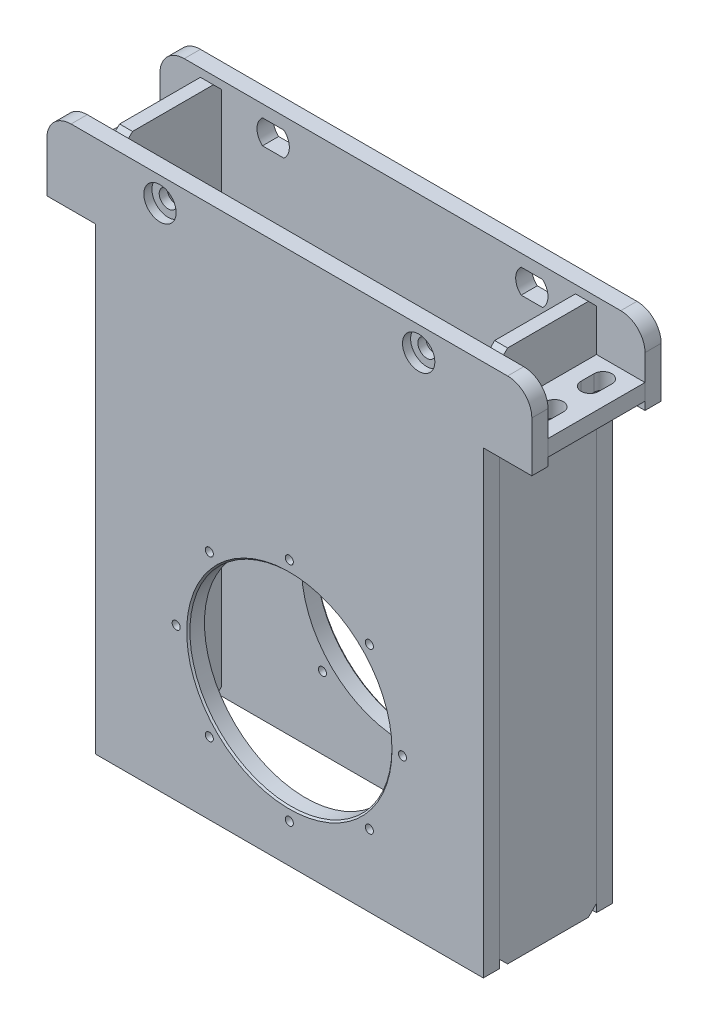
SolidWorks part; units mm, degrees
material "Plain carbon steel"
ref_plane "Front Plane" through (0, 0, 0) normal (0, 0, 1) x (1, 0, 0)
ref_plane "Top Plane" through (0, 0, 0) normal (0, 1, 0) x (1, 0, 0)
ref_plane "Right Plane" through (0, 0, 0) normal (1, 0, 0) x (0, 0, -1)
sketch "Sketch1" plane through (0, 0, 0) normal (0, 0, 1) x (1, 0, 0)
  line L1 (-150, 165) -> (150, 165)
  line L2 (-150, 165) -> (-150, -165)
  line L3 (-150, -165) -> (150, -165)
  line L4 (150, 165) -> (150, -165)
  line L5 (-150, 165) -> (150, -165) construction
  line L6 (-150, -165) -> (150, 165) construction
  point P0 (0, 0)
  dimension "D1" = 300
  dimension "D2" = 330
extrude "Boss-Extrude1" add sketch "Sketch1" along normal blind 10
sketch "Sketch2" plane through (0, 0, 10) normal (0, 0, 1) x (1, 0, 0)
  line L0 (150, 165) -> (-150, 165) construction
  circle A0 centre (-80, 150) radius 7.5
  dimension "D2" = 15
  dimension "D3" = 15
  dimension "D1" = 80
extrude "Cut-Extrude1" cut sketch "Sketch2" against normal blind 10
pattern_linear "LPattern1" count 2 spacing 160 along (1, 0, 0) of "Cut-Extrude1"
sketch "Sketch12" plane through (0, 0, 10) normal (0, 0, 1) x (1, 0, 0)
  line L0 (-150, -165) -> (150, -165) construction
  line L1 (120, -165) -> (112, -165)
  line L2 (120, -165) -> (120, 165)
  line L3 (120, 165) -> (112, 165)
  line L4 (112, -165) -> (112, 165)
  line L5 (-120, -165) -> (-112, -165)
  line L6 (-120, -165) -> (-120, 165)
  line L7 (-120, 165) -> (-112, 165)
  line L8 (-112, -165) -> (-112, 165)
  dimension "D1" = 330
  dimension "D2" = 8
  dimension "D3" = 8
  dimension "D4" = 330
  dimension "D5" = 120
  dimension "D6" = 120
extrude "Boss-Extrude2" add sketch "Sketch12" along normal blind 60 separate body
sketch "Sketch13" plane through (0, 0, 70) normal (0, 0, 1) x (1, 0, 0)
  line L0 (-150, 165) -> (-150, -165) construction
  line L1 (150, -165) -> (-150, -165)
  line L2 (150, -165) -> (150, 150)
  line L3 (135, 165) -> (-135, 165)
  line L4 (-150, -165) -> (-150, 150)
  arc A0 (150, 150) -> (135, 165) centre (135, 150) ccw
  arc A1 (-135, 165) -> (-150, 150) centre (-135, 150) ccw
  circle A2 centre (80, 150) radius 7.5 construction
  circle A3 centre (-80, 150) radius 7.5 construction
  circle A4 centre (80, 150) radius 7.5
  circle A5 centre (-80, 150) radius 7.5
  point P11 (-150, 165)
  dimension "D2" = 15
  dimension "D1" = 330
extrude "Boss-Extrude3" add sketch "Sketch13" along normal blind 10 separate body
sketch "Sketch14" plane through (120, 0, 0) normal (1, 0, 0) x (0, 0, -1)
  line L0 (-70, -165) -> (-70, 165) construction
  line L1 (-70, 124) -> (-10, 124)
  line L2 (-70, 124) -> (-70, 134)
  line L3 (-70, 134) -> (-10, 134)
  line L4 (-10, 124) -> (-10, 134)
  line L5 (-10, -165) -> (-10, 165) construction
  line L6 (-80, 165) -> (-70, 165) construction
  dimension "D1" = 10
  dimension "D2" = 31
extrude "Boss-Extrude4" add sketch "Sketch14" along normal blind 30 separate body
sketch "Sketch26" plane through (0, 134, 0) normal (0, 1, 0) x (1, 0, 0)
  line L0 (135, -10) -> (135, -70) construction
  line L1 (150, -10) -> (120, -10) construction
  line L2 (150, -70) -> (120, -70) construction
  line L3 (135, -40) -> (157.7954, -40) construction
  line L4 (135, -21) -> (135, -29) construction
  line L5 (140.5, -21) -> (140.5, -29)
  line L6 (129.5, -21) -> (129.5, -29)
  line L7 (135, -59) -> (135, -51) construction
  line L8 (129.5, -59) -> (129.5, -51)
  line L9 (140.5, -59) -> (140.5, -51)
  circle A0 centre (135, -25) radius 5.5 construction
  circle A1 centre (135, -55) radius 5.5 construction
  arc A2 (140.5, -21) -> (129.5, -21) centre (135, -21) ccw
  arc A3 (129.5, -29) -> (140.5, -29) centre (135, -29) ccw
  arc A4 (129.5, -59) -> (140.5, -59) centre (135, -59) ccw
  arc A5 (140.5, -51) -> (129.5, -51) centre (135, -51) ccw
  circle A6 centre (135, -21) radius 9 construction
  point P14 (135, -25)
  point P20 (135, -55)
  dimension "D1" = 11
  dimension "D2" = 30
  dimension "D4" = 18
  dimension "D3" = 8
extrude "Cut-Extrude6" cut sketch "Sketch26" against normal up to surface (10 mm away) up to face at (135, 124, 40)
mirror "Mirror1" about plane through (0, 0, 0) normal (1, 0, 0) of bodies 134 119
fillet "Fillet1" radius 15 2 edges at (150, 165, 5) (-150, 165, 5)
sketch "Sketch3" plane through (0, 0, 0) normal (0, 0, 1) x (1, 0, 0)
  line L0 (-150, -165) -> (150, -165) construction
  line L1 (0, -165) -> (0, -71) construction
  line L2 (135, 165) -> (-135, 165) construction
  circle A0 centre (0, -71) radius 62.5
  dimension "D1" = 125
  dimension "D2" = 236
extrude "Cut-Extrude2" cut sketch "Sketch3" along normal blind 170
hole_wizard "M6 Tapped Hole1" positions "Sketch4" profile "Sketch5" tap size "M6" standard "GB"
sketch "Sketch4" plane through (0, 0, 10) normal (0, 0, 1) x (1, 0, 0)
  line L0 (0, -71) -> (70.5063, -71) construction
  line L3 (0, -71) -> (49.4975, -21.5025) construction
  point P0 (49.4975, -21.5025)
  dimension "D1" = 70
  dimension "D2" = 45
sketch "Sketch5" plane through (49.4975, -21.5025, 10) normal (1, 0, 0) x (0, -1, 0)
  line L0 (0, 0) -> (0, 18.5022)
  line L1 (0, 18.5022) -> (2.5, 17)
  line L2 (2.5, 17) -> (2.5, 0)
  line L5 (2.5, 0) -> (0, 0)
  line L10 (0, 18.5022) -> (-2.5, 17) construction
  line L11 (0, -6.35) -> (0, 107.95) construction
  dimension "螺纹孔钻头直径" = 5
  dimension "螺纹孔钻头深度" = 17
  dimension "导头角度" = 118
cosmetic thread "Hole thread1" parameters "D1"=12, "D2"=6
pattern_circular "CirPattern1" count 8 over 360 about axis through (0, -71, 0) along (0, 0, 1) of "M6 Tapped Hole1"
cosmetic thread "Hole thread2" parameters "D1"=12, "D2"=6
cosmetic thread "Hole thread3" parameters "D1"=12, "D2"=6
cosmetic thread "Hole thread4" parameters "D1"=12, "D2"=6
cosmetic thread "Hole thread5" parameters "D1"=12, "D2"=6
cosmetic thread "Hole thread6" parameters "D1"=12, "D2"=6
cosmetic thread "Hole thread7" parameters "D1"=12, "D2"=6
cosmetic thread "Hole thread8" parameters "D1"=12, "D2"=6
sketch "Sketch16" plane through (0, 0, 80) normal (0, 0, 1) x (1, 0, 0)
  line L0 (135, 165) -> (-135, 165) construction
  line L1 (150, -165) -> (120, -165)
  line L2 (150, -165) -> (150, 119)
  line L3 (150, 119) -> (120, 119)
  line L4 (120, -165) -> (120, 119)
  line L5 (-150, -165) -> (-120, -165)
  line L6 (-150, -165) -> (-150, 119)
  line L7 (-150, 119) -> (-120, 119)
  line L8 (-120, -165) -> (-120, 119)
  dimension "D1" = 30
  dimension "D2" = 30
  dimension "D3" = 46
  dimension "D4" = 46
extrude "Cut-Extrude3" cut sketch "Sketch16" against normal blind 141
hole_wizard "M6 Tapped Hole2" positions "Sketch19" profile "Sketch20" tap size "M6" standard "GB"
sketch "Sketch19" plane through (0, 0, 80) normal (0, 0, 1) x (1, 0, 0)
  line L0 (-70, -71) -> (0, -71) construction
  point P0 (-70, -71)
  dimension "D1" = 70
sketch "Sketch20" plane through (-70, -71, 80) normal (1, 0, 0) x (0, -1, 0)
  line L0 (0, 0) -> (0, 26.0022)
  line L1 (0, 26.0022) -> (2.5, 24.5)
  line L2 (2.5, 24.5) -> (2.5, 0)
  line L5 (2.5, 0) -> (0, 0)
  line L10 (0, 26.0022) -> (-2.5, 24.5) construction
  line L11 (0, -6.35) -> (0, 107.95) construction
  dimension "螺纹孔钻头直径" = 5
  dimension "螺纹孔钻头深度" = 24.5
  dimension "导头角度" = 118
cosmetic thread "Hole thread9" parameters "D1"=12, "D2"=6
pattern_circular "CirPattern2" count 8 over 360 about axis through (0, -71, 0) along (0, 0, 1) of "M6 Tapped Hole2"
cosmetic thread "Hole thread10" parameters "D1"=12, "D2"=6
cosmetic thread "Hole thread11" parameters "D1"=12, "D2"=6
cosmetic thread "Hole thread12" parameters "D1"=12, "D2"=6
cosmetic thread "Hole thread13" parameters "D1"=12, "D2"=6
cosmetic thread "Hole thread14" parameters "D1"=12, "D2"=6
cosmetic thread "Hole thread15" parameters "D1"=12, "D2"=6
cosmetic thread "Hole thread16" parameters "D1"=12, "D2"=6
sketch "Sketch21" plane through (0, 0, 0) normal (0, 0, -1) x (-1, 0, 0)
  circle A0 centre (-80, 150) radius 10
  dimension "D1" = 20
extrude "Cut-Extrude4" cut sketch "Sketch21" against normal blind 18
pattern_linear "LPattern2" count 2 spacing 160 along (-1, 0, 0) of "Cut-Extrude4"
sketch "Sketch22" plane through (0, 0, 80) normal (0, 0, 1) x (1, 0, 0)
  circle A0 centre (80, 150) radius 10
  circle A1 centre (-80, 150) radius 10
  dimension "D1" = 20
  dimension "D2" = 20
extrude "Cut-Extrude5" cut sketch "Sketch22" against normal blind 5
chamfer "Chamfer1" distance 1 angle 45 1 edges at (62.5, -71, 80)
chamfer "Chamfer2" distance 1 angle 45 1 edges at (62.5, -71, 0)
sketch "Sketch23" plane through (0, 0, 70) normal (0, 0, -1) x (-1, 0, 0)
  circle A0 centre (-80, 150) radius 5.5
  circle A1 centre (80, 150) radius 5.5
  circle A2 centre (-80, 150) radius 7.5 construction
  circle A3 centre (-80, 150) radius 7.5
  circle A4 centre (80, 150) radius 7.5 construction
  circle A5 centre (80, 150) radius 7.5
  dimension "D1" = 11
extrude "Boss-Extrude5" add sketch "Sketch23" against normal up to surface (5 mm away) up to face at (87.5, 150, 75)
sketch "Sketch24" plane through (0, 0, 0) normal (0, 0, -1) x (-1, 0, 0)
  line L1 (-93.5972, 142.5) -> (-66.4028, 142.5)
  line L2 (-93.5972, 142.5) -> (-93.5972, 157.5)
  line L3 (-93.5972, 157.5) -> (-66.4028, 157.5)
  line L4 (-66.4028, 142.5) -> (-66.4028, 157.5)
  line L5 (-93.5972, 142.5) -> (-66.4028, 157.5) construction
  line L6 (-93.5972, 157.5) -> (-66.4028, 142.5) construction
  line L7 (61.3571, 142.5) -> (98.6429, 142.5)
  line L8 (61.3571, 142.5) -> (61.3571, 157.5)
  line L9 (61.3571, 157.5) -> (98.6429, 157.5)
  line L10 (98.6429, 142.5) -> (98.6429, 157.5)
  line L11 (61.3571, 142.5) -> (98.6429, 157.5) construction
  line L12 (61.3571, 157.5) -> (98.6429, 142.5) construction
  circle A0 centre (-80, 150) radius 10 construction
  circle A1 centre (-80, 150) radius 10
  circle A2 centre (80, 150) radius 10
  circle A3 centre (80, 150) radius 10 construction
  point P0 (-80, 150)
  circle M11 centre (80, 150) radius 10
  circle M12 centre (-80, 150) radius 10
  dimension "D1" = 15
  dimension "D2" = 15
extrude "Boss-Extrude6" add sketch "Sketch24" against normal up to surface (10 mm away) contours L9 M11 | L7 M11 | L3 M12 | L1 M12 up to face at (-70, 150, 10)
chamfer "Chamfer3" distance 5 angle 45 4 edges at (-116, -165, 10) (-116, -165, 70) (-116, 165, 10) (-116, 165, 70)
chamfer "Chamfer4" distance 5 angle 45 4 edges at (116, -165, 10) (116, -165, 70) (116, 165, 10) (116, 165, 70)
